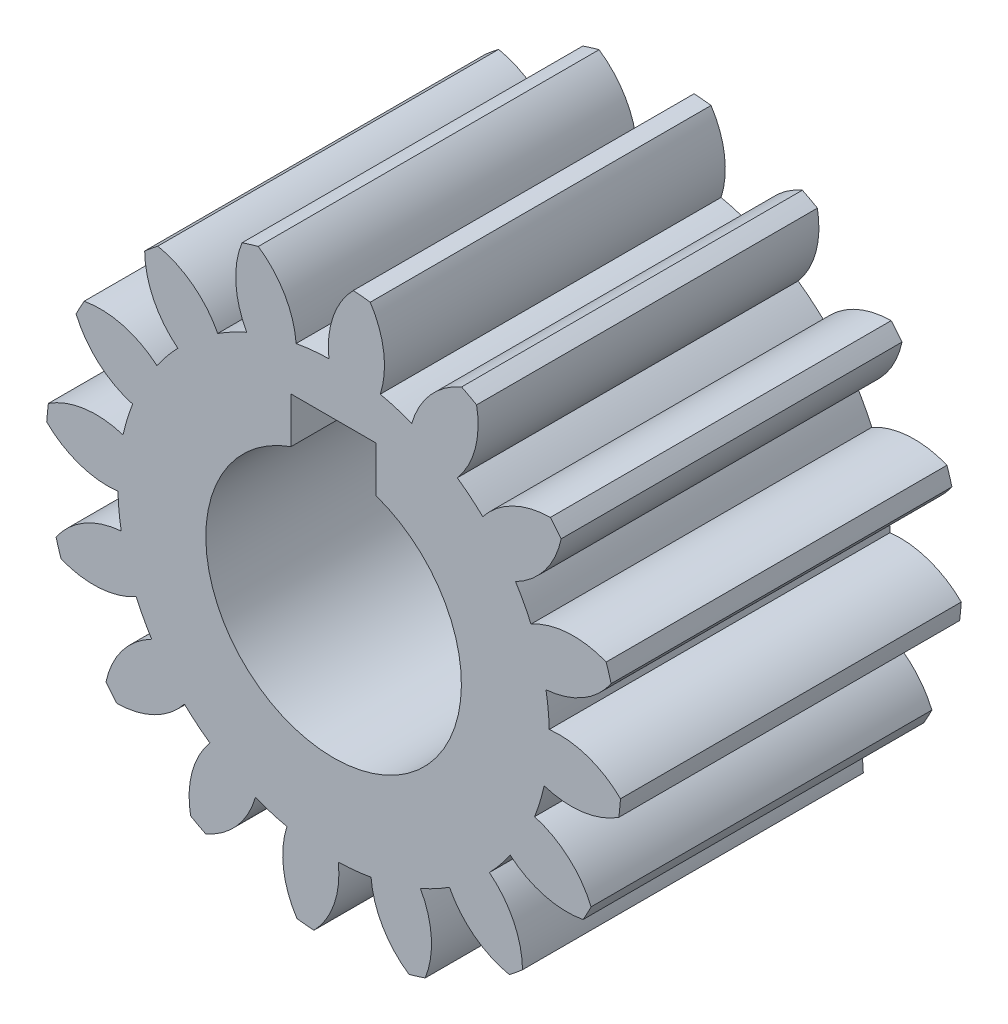
SolidWorks part; units mm, degrees
ref_plane "Front Plane" through (0, 0, 0) normal (0, 0, 1) x (1, 0, 0)
ref_plane "Top Plane" through (0, 0, 0) normal (0, 1, 0) x (1, 0, 0)
ref_plane "Right Plane" through (0, 0, 0) normal (1, 0, 0) x (0, 0, -1)
other "Configuration Table"
sketch "Sketch1" plane through (0, 0, 0) normal (0, 0, 1) x (1, 0, 0)
  circle A0 centre (0, 0) radius 10.125
  dimension "D1" = 20.25
extrude "Boss-Extrude1" add sketch "Sketch1" along normal blind 16
sketch "Sketch2" plane through (0, 0, 16) normal (0, 0, 1) x (1, 0, 0)
  line L0 (0, 0) -> (0, 13.5) construction
  line L1 (0, 0) -> (4.6173, 12.6859) construction
  line L2 (0, 0) -> (1.5188, 15.4209) construction
  line L3 (0, 12) -> (3.8567, 10.5963) construction
  circle A0 centre (0, 0) radius 12 construction
  circle A1 centre (0, 0) radius 13.5
  arc A2 (0.9248, 13.4683) -> (-0.2201, 10.1226) centre (3.8567, 10.5963) ccw
  circle A3 centre (0, 0) radius 10.125 construction
  circle A4 centre (0, 0) radius 10.125
  arc A5 (1.7205, 13.3899) -> (2.1907, 9.8852) centre (-1.7154, 11.1451) cw
  dimension "D1" = 24
  dimension "D2" = 27
  dimension "D3" = 20
  dimension "D4" = 5.625
extrude "Boss-Extrude2" add sketch "Sketch2" against normal blind 16 contours A5 A1 A2 A4
pattern_circular "CirPattern1" count 16 over 360 about axis through (0, 0, 0) along (0, 0, 1) of "Boss-Extrude2"
sketch "Sketch3" plane through (0, 0, 16) normal (0, 0, 1) x (1, 0, 0)
  line L1 (-2, 4.2) -> (2, 4.2)
  line L2 (-2, 4.2) -> (-2, 7.8)
  line L3 (-2, 7.8) -> (2, 7.8)
  line L4 (2, 4.2) -> (2, 7.8)
  line L5 (-2, 4.2) -> (2, 7.8) construction
  line L6 (-2, 7.8) -> (2, 4.2) construction
  circle A0 centre (0, 0) radius 6
  point P3 (0, 6)
  dimension "D2" = 12
  dimension "D1" = 7.8
  dimension "D3" = 4
extrude "Cut-Extrude1" cut sketch "Sketch3" against normal blind 16 contours L2 L3 L4 L1 | A0
